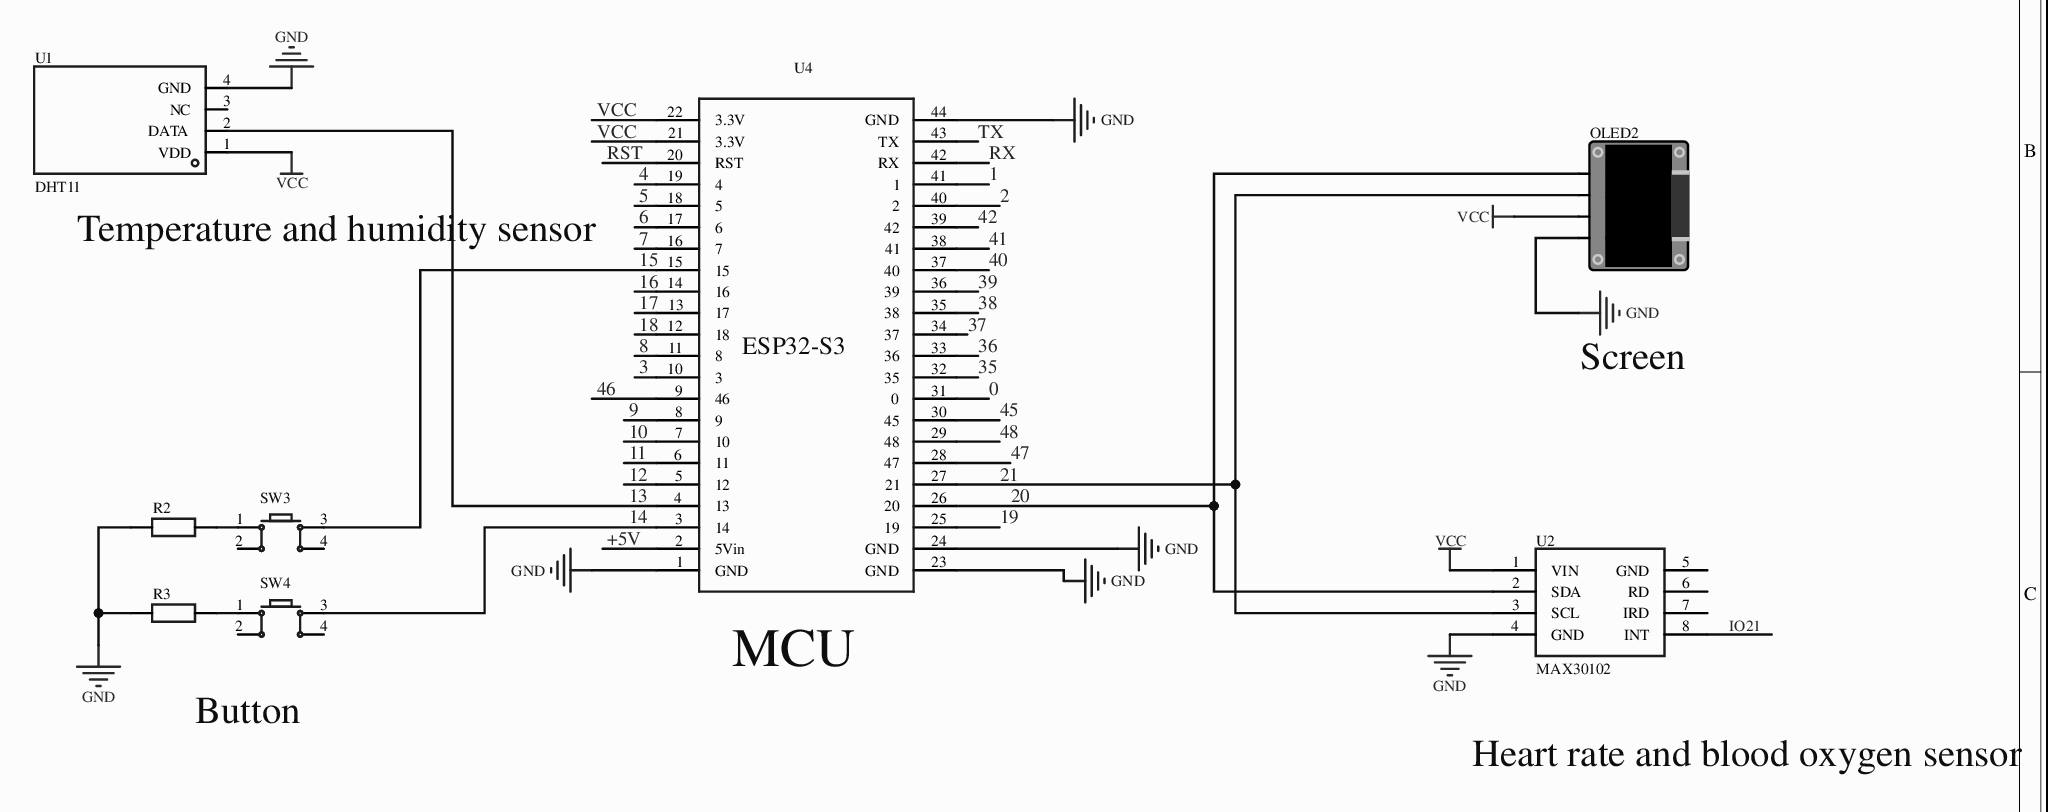
[diagram p0: MISC61243-3.schdoc]
# Altium project MISC61243-2.PrjPcb
1 sheet, 8 parts. Net scope: global (net labels, ports and power ports of the same name join across sheets).
Board file: MISC61243.pcbdoc

## Sheet MISC61243-3.schdoc
size 297 x 209 mm; Version: V1.0; @Project Name: MISC61243; @Page Count: 1; @Update Date: 2026-04-29; @Create Date: 2026-04-29; @Schematic Name: MISC61243; @Page No: 1; @Create Time: 23:22:16; @Update Time: 17:32:40; @Board Name: MISC61243

### Parts
OLED2  (no value)  [0.96OLED_4P]
R2  10K  [R0603]  (value not drawn)
R3  10K  [R0603]  (value not drawn)
SW3  (no value)  [SW-TH_4P-L6.0-W6.0-P4.50-LS6.5]
SW4  (no value)  [SW-TH_4P-L6.0-W6.0-P4.50-LS6.5]
U1  DHT11  [SENSOR-TH_DHT11]
U2  MAX30102  [MAX30102]
U4  NO  [ESP32S3]  (value not drawn)

### Nets
GND: OLED2.1(GND) R2.1 R3.1 U1.4(GND) U2.4(GND) U4.1(GND) U4.23(GND) U4.24(GND) U4.44(GND)
VCC: OLED2.2(VCC) U1.1(VDD) U2.1(VIN) U4.21(3.3V) U4.22(3.3V)
0: U4.31(0)
1: U4.41(1)
2: U4.40(2)
3: U4.10(3)
4: U4.19(4)
5: U4.18(5)
6: U4.17(6)
7: U4.16(7)
8: U4.11(8)
9: U4.8(9)
10: U4.7(10)
11: U4.6(11)
12: U4.5(12)
13: U1.2(DATA) U4.4(13)
14: SW4.3 U4.3(14)
15: SW3.3 U4.15
16: U4.14(16)
17: U4.13(17)
18: U4.12(18)
19: U4.25(19)
20: OLED2.4(SDA) U2.2(SDA) U4.26(20)
21: OLED2.3(SCL) U2.3(SCL) U4.27(21)
35: U4.32(35)
36: U4.33(36)
37: U4.34(37)
38: U4.35(38)
39: U4.36(39)
40: U4.37(40)
41: U4.38(41)
42: U4.39(42)
45: U4.30(45)
46: U4.9(46)
47: U4.28(47)
48: U4.29(48)
+5V: U4.2(5Vin)
IO21: U2.8(INT)
RST: U4.20(RST)
RX: U4.42(RX)
TX: U4.43(TX)
NetR2_2: R2.2 SW3.1
NetR3_2: R3.2 SW4.1

Not connected (* = marked no-connect by the designer): SW3 2 4; SW4 2 4; U1 3(NC); U2 5(GND) 6(RD) 7(IRD)

### Notes on the sheet
- (near U4) Temperature and humidity sensor
- Screen
- Button
- (near U4) MCU
- Heart rate and blood oxygen sensor

### Library data of the parts
OLED2 = 0.96OLED模块_4P: Symbol: 0.96OLED module_4P; 3D Model: 79c000fdb68d45a296c2e9bedf4f9055; 3D Model Transform: 1393.69792,1318.895,0,0,0,0,0,-560.079,-137.795; ConvertToPcb: yes; Device: 0.96OLED module_4P; Supplier Footprint: 插件; AddInBom: yes; FootprintName: 0.96OLED_4P; ModelName: 0.96OLED_4P
R2 R3 = Res_0603: Symbol: Resistor; 3D Model: fc143cca1e79419f9cd78b61e9279f080819f05c4eef4c71ace90d822a990e87; 3D Model Transform: 31.8897,63.7794,0,90,0,0,0,0,0; ConvertToPcb: yes; Device: Res_0603; Supplier Footprint: 0603; Value: 10K; AddInBom: yes; FootprintName: R0603; ModelName: R0603
SW3 SW4 = Key_TH_6x6x6: Contact current:50mA; Rated voltage (DC):12V; Insulation resistance:100MΩ; Circuit structure: SPST; Mounting: through-hole; Button shape: round button; Button/cap colour: black; Actuation force: 260gf@±30gf; Operating temperature: -25℃~+70℃; Pin style: PC pin; Switch length: 6mm; Switch width: 6mm; Switch height: 6mm; With bracket: no;; Symbol: Tactile switch; AddInBom: yes; ModelId: 20eee248bc684ccd8cbdbb1d0d91ec6f0819f05c4eef4c71ace90d822a990e87; ModelName: SW-TH_4P-L6.0-W6.0-H5.0-LS6.5-P4.50; ModelTransform: 236.22,323.03,0,90,0,0,0,0,-137.795; Device: Key_TH_6x6x6; FootprintName: SW-TH_4P-L6.0-W6.0-P4.50-LS6.5; ConvertToPcb: yes; Supplier Footprint: 插件
U1 = DHT11: New capacitive digital temperature and humidity sensor; old model discontinued; 16.1x12.6x5.8mm; Manufacturer: 广州奥松; AddInBom: yes; ModelId: 6dde47d4d8bf4fa598dffcc067449c1d; ModelTransform: 236.25937,492.125,0,270,0,0,0,-11.811,-196.85; Symbol: DHT11; Device: DHT11; LCSC Part Name: 新款电容式数字温湿度传感器,老款已停产16.1x12.6x5.8mm DHT11  电容式传感器; SupplierPart: C117051; ManufacturerPart: DHT11; Supplier Footprint: SIP-4; JLCPCB Part Class: Extended library; Datasheet: https://atta.szlcsc.com/upload/public/pdf/source/20170703/1499081238365.pdf; Supplier: LCSC; ConvertToPcb: yes; FootprintName: SENSOR-TH_DHT11; ModelName: SENSOR-TH_DHT11
U2 = MAX30102: AddInBom: yes; Symbol: MAX30102; Device: MAX30102; ConvertToPcb: yes; FootprintName: MAX30102
U4 = NO: Add into BOM: yes; Symbol: NO; Device: NO; Convert to PCB: yes; Origin Footprint: ESP32S3; FootprintName: ESP32S3